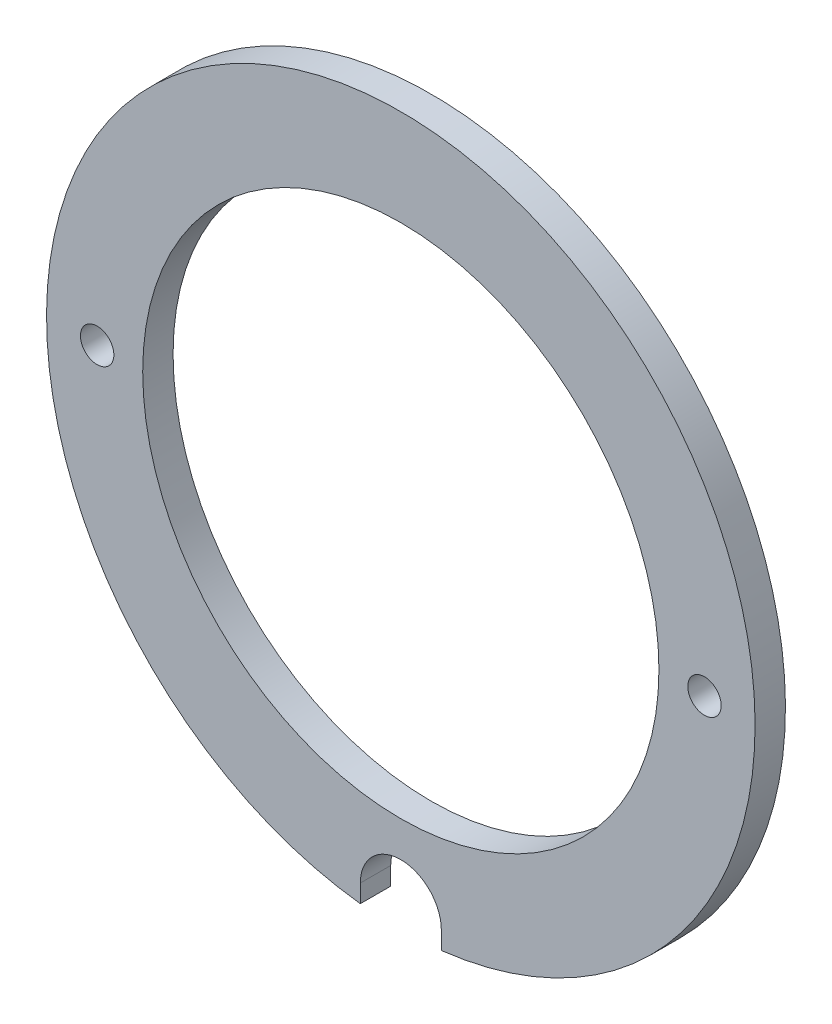
from build123d import *

# Parameters (mm, degrees)
SKETCH2_R           = 35
SKETCH2_R_2         = 25.5
BOSS_EXTRUDE1_DEPTH = 3
SKETCH3_R           = 4
CUT_EXTRUDE1_DEPTH  = 5
SKETCH8_W           = 8
SKETCH8_H           = 8.160533217
CUT_EXTRUDE3_DEPTH  = 50.588305073
SKETCH9_R           = 1.65
CUT_EXTRUDE4_DEPTH  = 50.588305073


with BuildPart() as part:
    # Sketch2 → Boss-Extrude1 (new body)
    with BuildSketch(Plane.XY):
        Circle(SKETCH2_R)
        Circle(SKETCH2_R_2, mode=Mode.SUBTRACT)
    extrude(amount=BOSS_EXTRUDE1_DEPTH)

    # Sketch3 → Cut-Extrude1 (cut)
    with BuildSketch(Plane(origin=(0, 0, 0), x_dir=(-1, 0, 0), z_dir=(0, 0, -1))):
        with Locations((0, -33)):
            Circle(SKETCH3_R)
    extrude(amount=-CUT_EXTRUDE1_DEPTH, mode=Mode.SUBTRACT)

    # Sketch8 → Cut-Extrude3 (cut, through all)
    with BuildSketch(Plane.XY.offset(3)):
        with Locations((0, -37.080266608)):
            Rectangle(SKETCH8_W, SKETCH8_H)
    extrude(amount=-CUT_EXTRUDE3_DEPTH, mode=Mode.SUBTRACT)

    # Sketch9 → Cut-Extrude4 (cut, through all)
    with BuildSketch(Plane.XY.offset(3)):
        with Locations((30, 0)):
            Circle(SKETCH9_R)
        with Locations(Location((-30, 0, 0), (0, 0, 180))):
            Circle(SKETCH9_R)
    extrude(amount=-CUT_EXTRUDE4_DEPTH, mode=Mode.SUBTRACT)


solid = part.part
